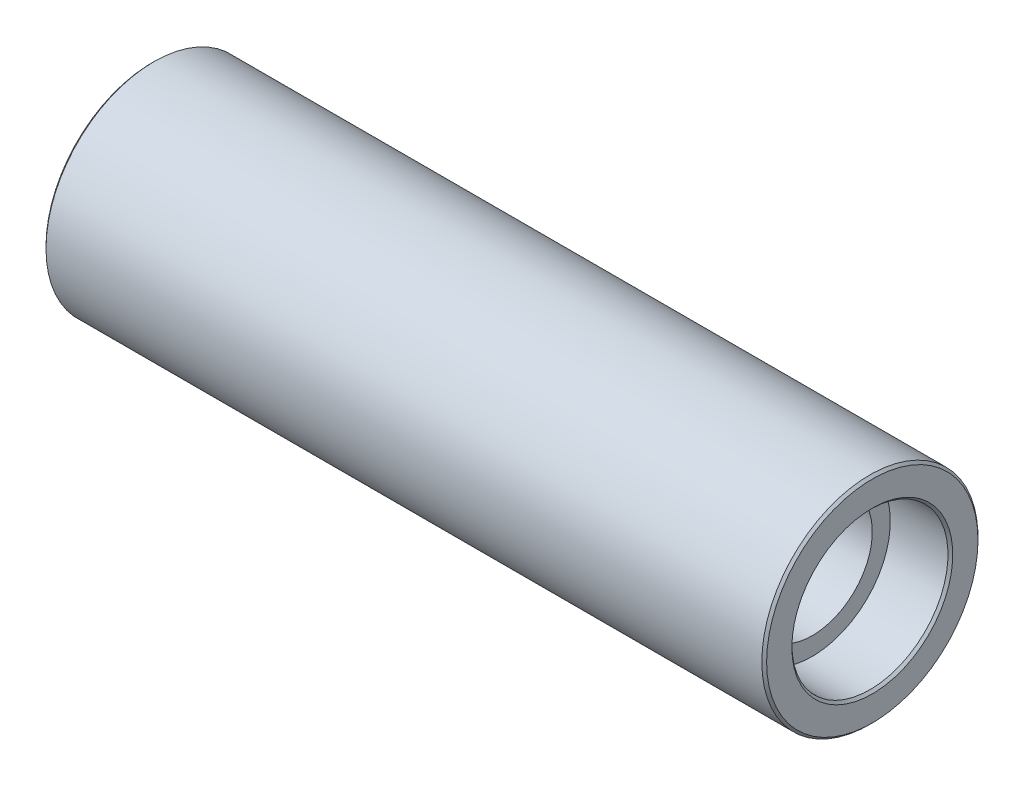
SolidWorks part; units mm, degrees
ref_plane "Front Plane" through (0, 0, 0) normal (0, 0, 1) x (1, 0, 0)
ref_plane "Top Plane" through (0, 0, 0) normal (0, 1, 0) x (1, 0, 0)
ref_plane "Right Plane" through (0, 0, 0) normal (1, 0, 0) x (0, 0, -1)
sketch "Sketch1" plane through (0, 0, 0) normal (0, 0, 1) x (1, 0, 0)
  line L0 (0, 0) -> (158.1254, 0) construction
  line L1 (0, 9) -> (60, 9)
  line L2 (60, 9) -> (60, 6.5)
  line L3 (60, 6.5) -> (55, 6.5)
  line L4 (55, 6.5) -> (55, 5)
  line L5 (55, 5) -> (5, 5)
  line L6 (5, 5) -> (5, 6.5)
  line L7 (5, 6.5) -> (0, 6.5)
  line L8 (0, 6.5) -> (0, 9)
  dimension "D1" = 60
  dimension "D2" = 10
  dimension "D3" = 13
  dimension "D4" = 5
  dimension "D5" = 18
revolve "Revolve1" add sketch "Sketch1" angle 360 about L0
chamfer "Chamfer1" distance 0.2 angle 45 4 edges at (0, 0, 9) (0, 0, 6.5) (60, 0, 9) (60, 0, 6.5)
